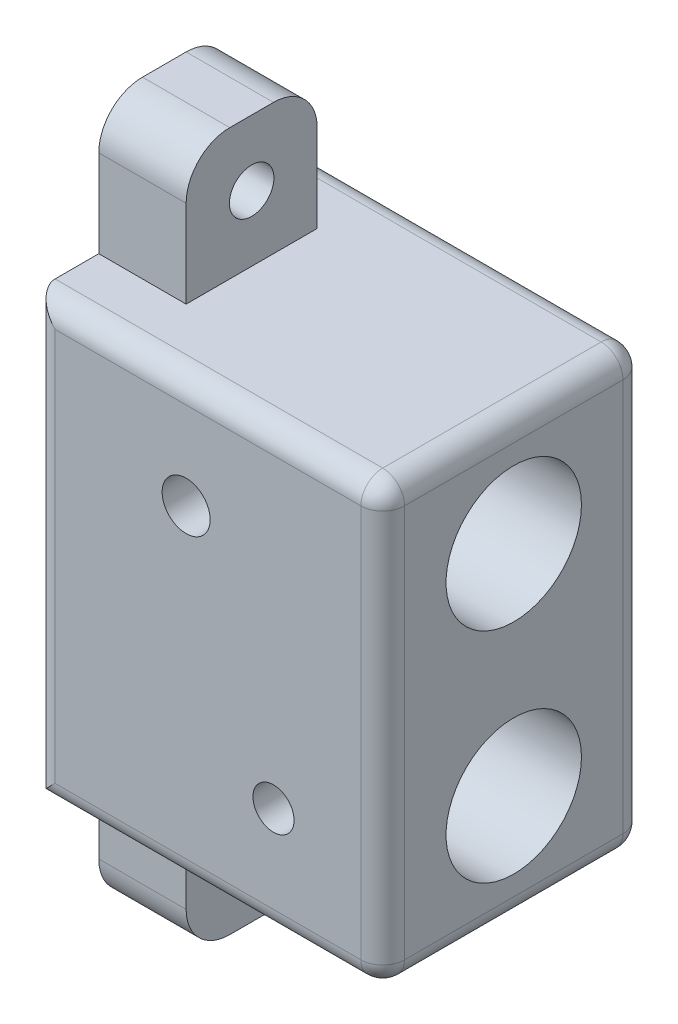
from build123d import *

# Parameters (mm, degrees)
BOSS_EXTRUDE1_DEPTH = 100
SKETCH2_R           = 15.5
CUT_EXTRUDE1_DEPTH  = 70
SKETCH3_R           = 5.1
CUT_EXTRUDE2_DEPTH  = 70
SKETCH4_R           = 5.5
SKETCH4_R_2         = 4.705316684
CUT_EXTRUDE3_DEPTH  = 70
SKETCH5_R           = 5.1
BOSS_EXTRUDE2_DEPTH = 20
SKETCH6_W           = 20
SKETCH6_H           = 100
CUT_EXTRUDE4_DEPTH  = 20
FILLET1_R           = 5


with BuildPart() as part:
    # Sketch1 → Boss-Extrude1 (new body)
    with BuildSketch(Plane(origin=(0, 0, 0), x_dir=(1, 0, 0), z_dir=(0, 1, 0))):
        Polygon((0, 20), (20, 20), (20, 0), (80, 0), (80, -60), (0, -60), (0, 0), align=None)
    extrude(amount=BOSS_EXTRUDE1_DEPTH)

    # Sketch2 → Cut-Extrude1 (cut)
    with BuildSketch(Plane(origin=(80, 0, 0), x_dir=(0, 0, -1), z_dir=(1, 0, 0))):
        with Locations((-30, 75)):
            Circle(SKETCH2_R)
        with Locations((-30, 25)):
            Circle(SKETCH2_R)
    extrude(amount=-CUT_EXTRUDE1_DEPTH, mode=Mode.SUBTRACT)

    # Sketch3 → Cut-Extrude2 (cut)
    with BuildSketch(Plane(origin=(20, 0, 0), x_dir=(0, 0, -1), z_dir=(1, 0, 0))):
        with Locations((10, 87.5)):
            Circle(SKETCH3_R)
        with Locations((10, 12.5)):
            Circle(SKETCH3_R)
        with Locations((10, 50)):
            Circle(SKETCH3_R)
    extrude(amount=-CUT_EXTRUDE2_DEPTH, mode=Mode.SUBTRACT)

    # Sketch4 → Cut-Extrude3 (cut)
    with BuildSketch(Plane(origin=(0, 0, 0), x_dir=(-1, 0, 0), z_dir=(0, 0, -1))):
        with Locations((-35, 75)):
            Circle(SKETCH4_R)
        with Locations((-55, 25)):
            Circle(SKETCH4_R_2)
    extrude(amount=-CUT_EXTRUDE3_DEPTH, mode=Mode.SUBTRACT)

    # Sketch5 → Boss-Extrude2 (add)
    with BuildSketch(Plane.ZY):
        with BuildLine():
            Line((35, 130), (25, 130))
            ThreePointArc((25, 130), (17.928932188, 127.071067812), (15, 120))
            Line((15, 120), (15, -20))
            ThreePointArc((15, -20), (17.928932188, -27.071067812), (25, -30))
            Line((25, -30), (35, -30))
            ThreePointArc((35, -30), (42.071067812, -27.071067812), (45, -20))
            Line((45, -20), (45, 120))
            ThreePointArc((45, 120), (42.071067812, 127.071067812), (35, 130))
        make_face()
        with Locations((30, -15)):
            Circle(SKETCH5_R, mode=Mode.SUBTRACT)
        with Locations((30, 115)):
            Circle(SKETCH5_R, mode=Mode.SUBTRACT)
    extrude(amount=-BOSS_EXTRUDE2_DEPTH)

    # Sketch6 → Cut-Extrude4 (cut)
    with BuildSketch(Plane(origin=(20, 0, 0), x_dir=(0, 0, -1), z_dir=(1, 0, 0))):
        with Locations((10, 50)):
            Rectangle(SKETCH6_W, SKETCH6_H)
    extrude(amount=-CUT_EXTRUDE4_DEPTH, mode=Mode.SUBTRACT)

    # Fillet1
    fillet1_edges = [part.edges().sort_by_distance(p)[0] for p in [
        (80, 100, 30),
        (80, 50, 0),
        (80, 50, 60),
        (0, 50, 60),
        (40, 100, 0),
        (0, 50, 0),
        (40, 100, 60),
        (40, 0, 0),
        (80, 0, 30),
        (40, 0, 60),
    ]]
    fillet(fillet1_edges, radius=FILLET1_R)


solid = part.part
